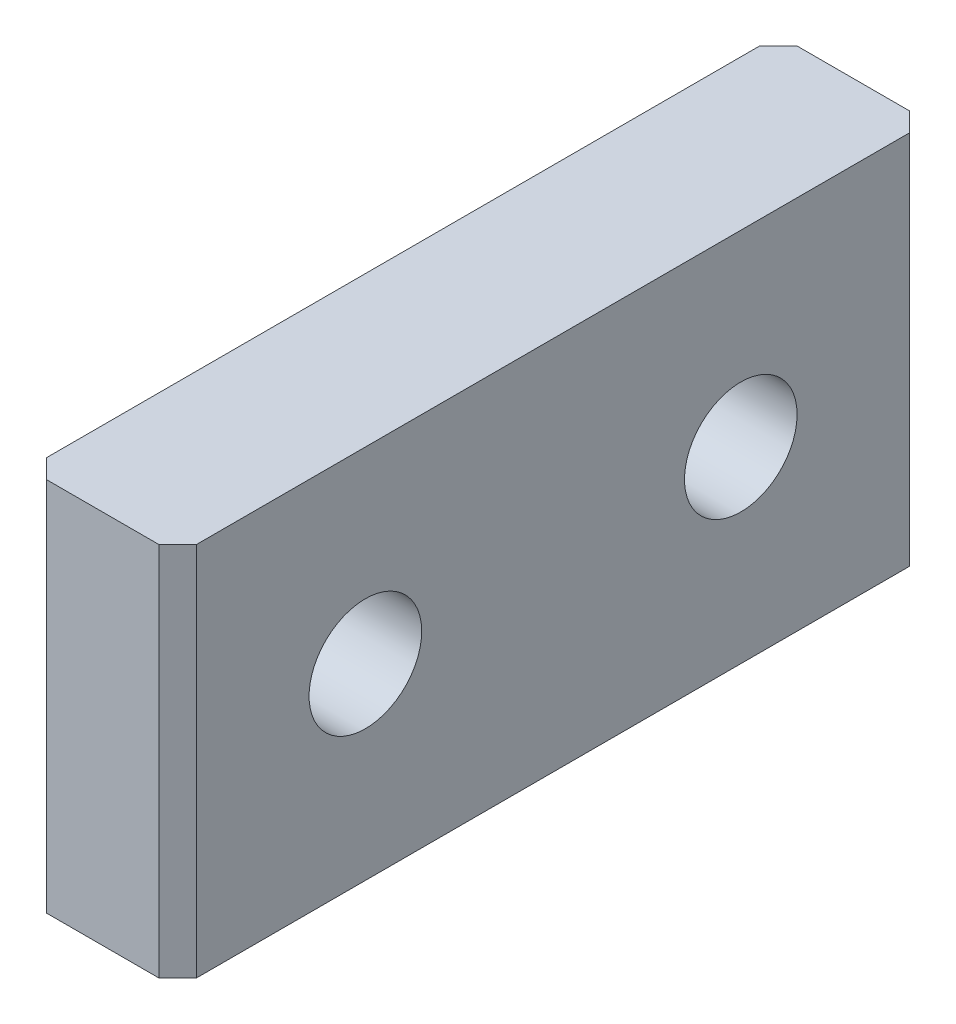
SolidWorks part; units mm, degrees
material "Q235-A"
ref_plane "Front Plane" through (0, 0, 0) normal (0, 0, 1) x (1, 0, 0)
ref_plane "Top Plane" through (0, 0, 0) normal (0, 1, 0) x (1, 0, 0)
ref_plane "Right Plane" through (0, 0, 0) normal (1, 0, 0) x (0, 0, -1)
sketch "Sketch1" plane through (0, 0, 0) normal (0, 1, 0) x (1, 0, 0)
  line L1 (0, 0) -> (8, 0)
  line L2 (0, 0) -> (0, -40)
  line L3 (0, -40) -> (8, -40)
  line L4 (8, 0) -> (8, -40)
  dimension "D1" = 8
  dimension "D2" = 40
extrude "Boss-Extrude1" add sketch "Sketch1" along normal blind 20
chamfer "Chamfer1" distance 1 angle 45 4 edges at (0, 10, 0) (8, 10, 0) (0, 10, 40) (8, 10, 40)
sketch "Sketch2" plane through (8, 0, 0) normal (1, 0, 0) x (0, 0, -1)
  line L0 (-30, 10) -> (-10, 10) construction
  line L1 (-20, 10) -> (-20, 0) construction
  line L2 (-39, 0) -> (-1, 0) construction
  circle A0 centre (-30, 10) radius 3
  circle A1 centre (-10, 10) radius 3
  dimension "D1" = 6
  dimension "D2" = 6
  dimension "D3" = 10
  dimension "D4" = 20
extrude "Cut-Extrude1" cut sketch "Sketch2" against normal through all
